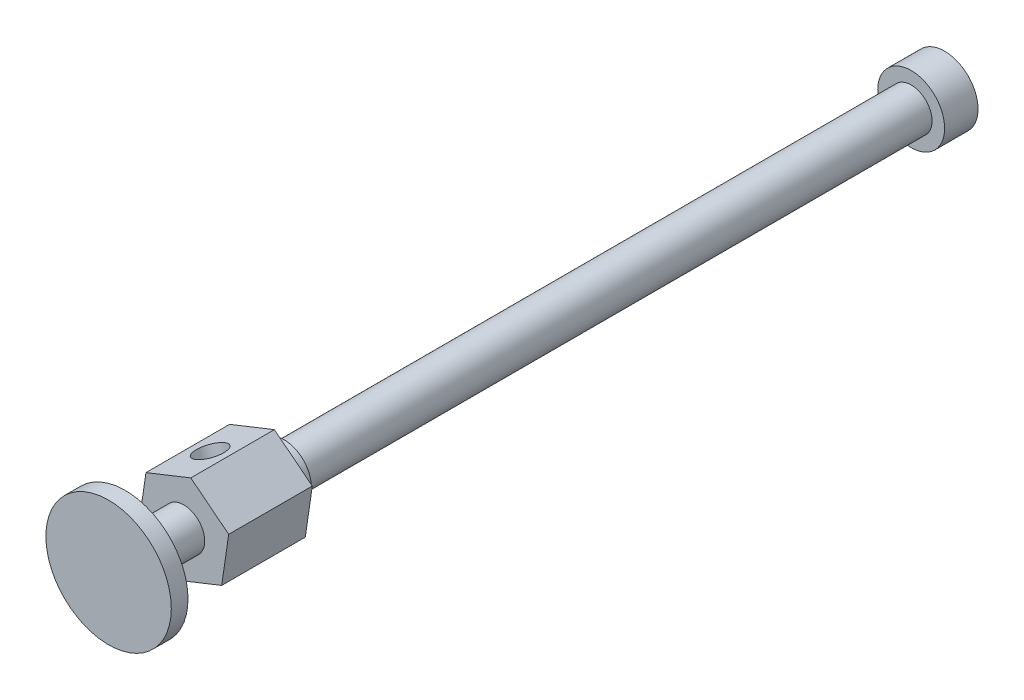
from build123d import *

# Parameters (mm, degrees)
SKETCH2_R           = 2.5
BOSS_EXTRUDE1_DEPTH = 100
SKETCH3_R           = 4
BOSS_EXTRUDE2_DEPTH = 4
SKETCH4_R           = 7.5
BOSS_EXTRUDE3_DEPTH = 2
BOSS_EXTRUDE4_DEPTH = 10
SKETCH6_R           = 3.25
BOSS_EXTRUDE5_DEPTH = 2
SKETCH7_R           = 1.75
CUT_EXTRUDE1_DEPTH  = 2


with BuildPart() as part:
    # Sketch2 → Boss-Extrude1 (new body)
    with BuildSketch(Plane.XY):
        with Locations((20.609067119, -9.310698144)):
            Circle(SKETCH2_R)
    extrude(amount=BOSS_EXTRUDE1_DEPTH)

    # Sketch3 → Boss-Extrude2 (add)
    with BuildSketch(Plane(origin=(0, 0, 0), x_dir=(-1, 0, 0), z_dir=(0, 0, -1))):
        with Locations((-20.609067119, -9.310698144)):
            Circle(SKETCH3_R)
    extrude(amount=-BOSS_EXTRUDE2_DEPTH)

    # Sketch4 → Boss-Extrude3 (add)
    with BuildSketch(Plane.XY.offset(100)):
        with Locations((20.609067119, -9.310698144)):
            Circle(SKETCH4_R)
    extrude(amount=-BOSS_EXTRUDE3_DEPTH)

    # Sketch5 → Boss-Extrude4 (add)
    with BuildSketch(Plane(origin=(0, 0, 91), x_dir=(-1, 0, 0), z_dir=(0, 0, -1))):
        Polygon((-16.079485871, -5.730722299), (-21.444626522, -3.597977792), (-25.97420777, -7.177953637), (-25.138648367, -12.890673989), (-19.773507717, -15.023418496), (-15.243926469, -11.443442651), align=None)
    extrude(amount=BOSS_EXTRUDE4_DEPTH)

    # Sketch6 → Boss-Extrude5 (add)
    with BuildSketch(Plane(origin=(0, 0, 81), x_dir=(-1, 0, 0), z_dir=(0, 0, -1))):
        with Locations((-20.609067119, -9.310698144)):
            Circle(SKETCH6_R)
    extrude(amount=BOSS_EXTRUDE5_DEPTH)

    # Sketch7 → Cut-Extrude1 (cut)
    with BuildSketch(Plane(origin=(4.161383334, -10.468392636, 0), x_dir=(0.9292696196810543, 0.3694021845331033, 0), z_dir=(-0.3694021845331033, 0.9292696196810543, 0))):
        with Locations(Location((15.71198773, -86, 0), (0, 0, 180))):
            Circle(SKETCH7_R)
    extrude(amount=-CUT_EXTRUDE1_DEPTH, mode=Mode.SUBTRACT)


solid = part.part
